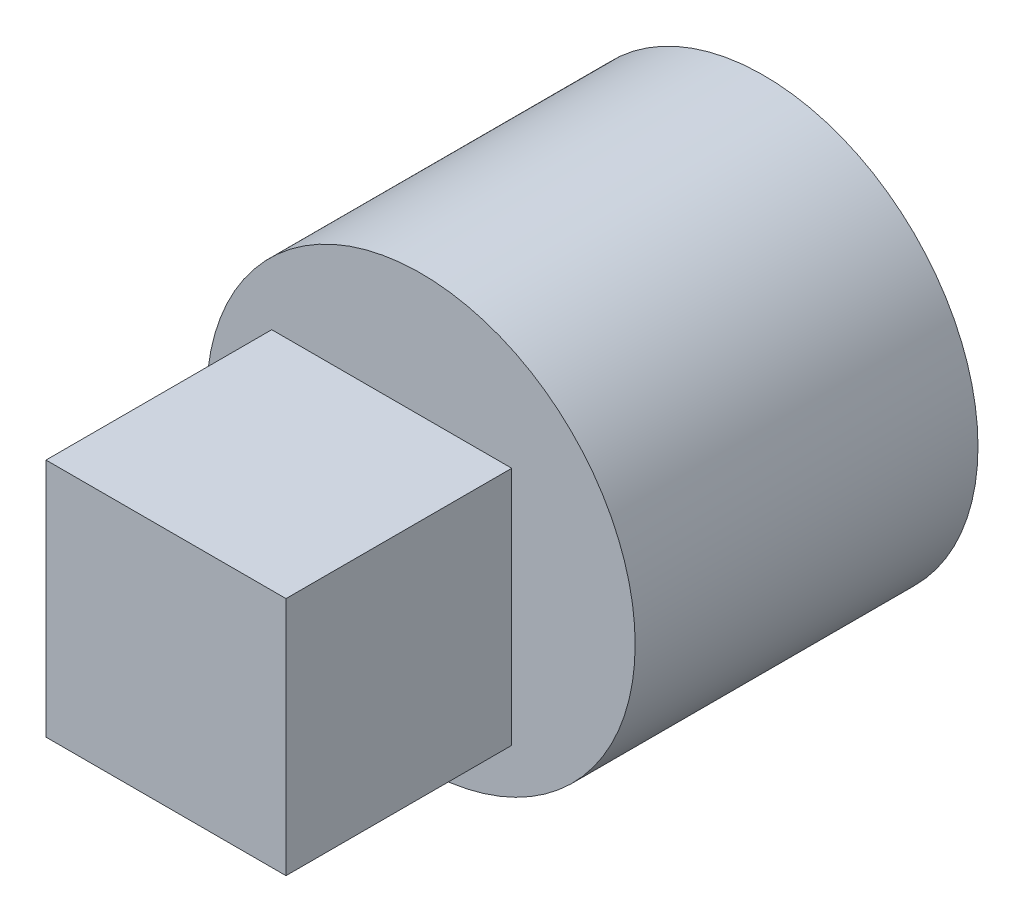
SolidWorks part; units mm, degrees
ref_plane "前视基准面" through (0, 0, 0) normal (0, 0, 1) x (1, 0, 0)
ref_plane "上视基准面" through (0, 0, 0) normal (0, 1, 0) x (1, 0, 0)
ref_plane "右视基准面" through (0, 0, 0) normal (1, 0, 0) x (0, 0, -1)
other "Configuration Table"
sketch "草图1" plane through (0, 0, 0) normal (0, 0, 1) x (1, 0, 0)
  circle A0 centre (0, 0) radius 12.5
  dimension "D1" = 25
extrude "凸台-拉伸1" add sketch "草图1" along normal blind 20
sketch "草图2" plane through (0, 0, 20) normal (0, 0, 1) x (1, 0, 0)
  line L1 (-4.25, -4.25) -> (4.25, -4.25)
  line L2 (-4.25, -4.25) -> (-4.25, 4.25)
  line L3 (-4.25, 4.25) -> (4.25, 4.25)
  line L4 (4.25, -4.25) -> (4.25, 4.25)
  line L5 (-4.25, -4.25) -> (4.25, 4.25) construction
  line L6 (-4.25, 4.25) -> (4.25, -4.25) construction
  point P0 (0, 0)
  dimension "D1" = 8.5
  dimension "D2" = 8.5
extrude "凸台-拉伸2" add sketch "草图2" along normal blind 1.7
sketch "草图3" plane through (0, 0, 21.7) normal (0, 0, 1) x (1, 0, 0)
  line L1 (-7, -7) -> (7, -7)
  line L2 (-7, -7) -> (-7, 7)
  line L3 (-7, 7) -> (7, 7)
  line L4 (7, -7) -> (7, 7)
  line L5 (-7, -7) -> (7, 7) construction
  line L6 (-7, 7) -> (7, -7) construction
  point P0 (0, 0)
  dimension "D1" = 14
  dimension "D2" = 14
extrude "凸台-拉伸3" add sketch "草图3" along normal blind 13.17
sketch "草图4" plane through (0, 0, 0) normal (0, 0, -1) x (-1, 0, 0)
  circle A0 centre (0, 0) radius 10
  dimension "D1" = 20
extrude "切除-拉伸1" cut sketch "草图4" against normal blind 15
chamfer "倒角1" distance 0.5 angle 45 4 edges at (0, -4.25, 20) (-4.25, 0, 20) (0, 4.25, 20) (4.25, 0, 20)
